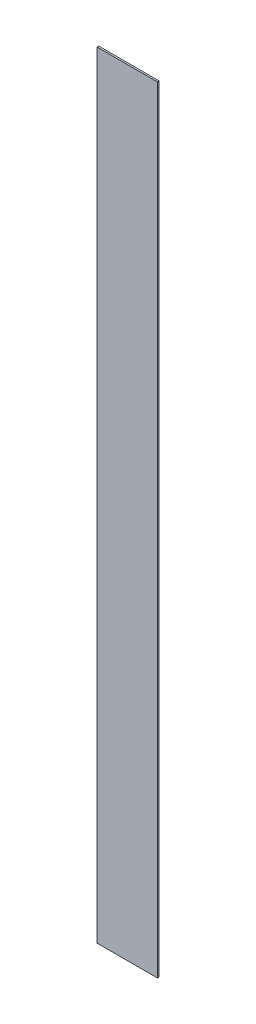
from build123d import *

# Parameters (mm, degrees)
SKETCH_1_W      = 180
SKETCH_1_H      = 2310
EXTRUDE_1_DEPTH = 5


with BuildPart() as part:
    # 草图1 → 凸台-拉伸1 (new body)
    with BuildSketch(Plane.XY):
        Rectangle(SKETCH_1_W, SKETCH_1_H)
    extrude(amount=EXTRUDE_1_DEPTH)


solid = part.part
